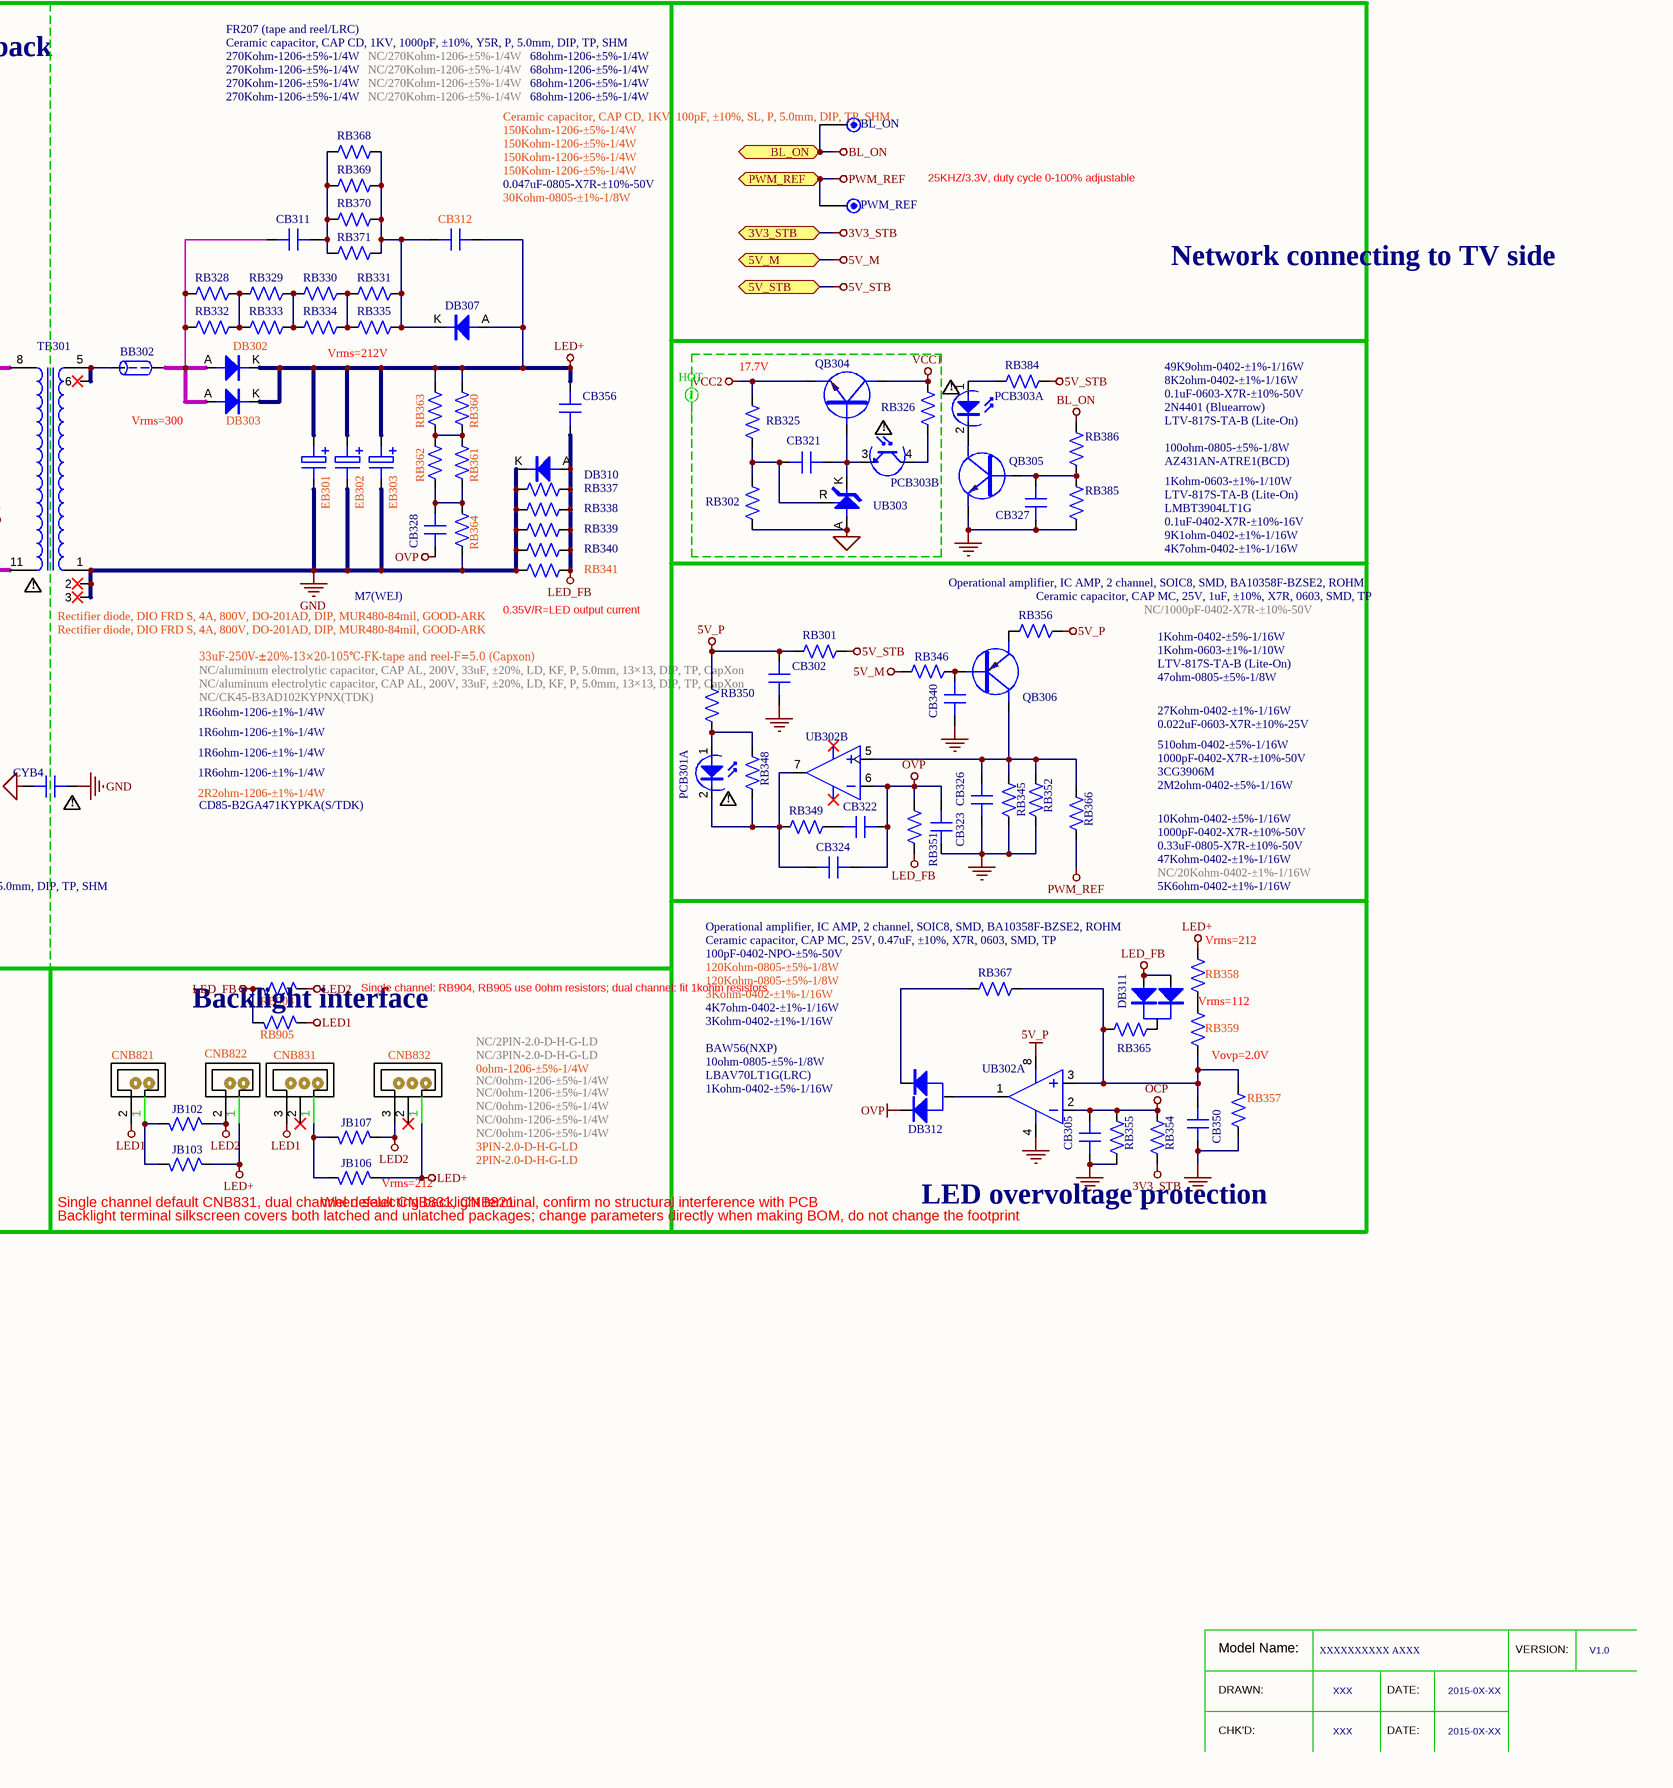
[diagram p0: PCBE84277.SchDoc, bottom right]
# Altium project MISC84277-14.PrjPCB (part 6 of 10)

## Sheet PCBE84277.SchDoc: MISC84277 (continued)

### Library data of the parts
BB101 = φ3.5×6.0×0.65mm-CP(编带/秀益达)-9-DAI: Through-hole ferrite bead
BB201 = Φ3.5×9.0×0.65mm(编带/秀益达)-DLAI: Through-hole ferrite bead
BB301 = φ3.5×6.0×0.65mm-CP(编带/秀益达)-DAI: Through-hole ferrite bead
BB302 = φ3.5×6.0×0.65mm-CP(编带/RY)-DLAI: Through-hole ferrite bead
CB2 CB3 = MPX450K474(散装/日精)-DHMI: CAP(474)
CB101 CB303 CB305 = 100pF-0402-NPO-±5%-50V-D
CB102 CB109 CB206 CB304 CB321 = 0.1uF-0603-X7R-±10%-50V-D: CAP
CB103 CB323 CB324 = 1000pF-0402-X7R-±10%-50V-D
CB110 CB340 = 1000pF-0402-X7R-±10%-50V-D: CAP
CB111 CB112 = 1uF-0805-X7R-±10%-25V-D: CAP
CB113 = 220PF-0805-NPO-±10%-200V-D: CAP
CB114 CB306 = C242G472J20A201(编带/法拉)-DAI: CAP
CB116 CB209 CB316 = 陶瓷电容,CAP CD,1KV,100pF,±10%,SL,P,5.0mm,DIP,TP,SHM-DHAI: CAP
CB118 = 1000pF-0805-NPO-±10%-200V-D: CAP
CB201 = 0.047uF-0603-X7R-±10%-25V-D
CB204 = 陶瓷电容,CAP CD,1KV,4700pF,±20%,Y5U,P,5.0mm,DIP,TP,SHM-DHAI
CB205 = 220pF-0402-NPO-±5%-50V-D
CB211 CB312 = CC45SL3AD470JYPNA(TDK)-DHAI: CAP
CB212 = 0.22uF-0805-X7R-±10%-50V-D
CB221 CB301 = 4700pF-0402-X7R-±10%-50V-D
CB302 = 陶瓷电容,CAP MC,25V,1uF,±10%,X7R,0603,SMD,TP-D: CAP
CB311 = CAP CD,1KV,1000pF,±10%,Y5R,P,5.0mm,DIP,TP,SHM-DHAI: CAP
CB322 = 0.022uF-0603-X7R-±10%-25V-D
CB326 = 0.33uF-0805-X7R-±10%-50V-D: C
CB327 CB951 = 0.1uF-0402-X7R-±10%-16V-D: CAP
CB328 = 0.047uF-0805-X7R-±10%-50V-D
CB350 = 0.47uF-0603-X5R-±10%-16V-D
CB356 = CK45-B3AD102KYPNX(TDK)-DHAI: CAP
CNB1 = 连接插座,connect jack,2Pin,D7.92,L,SNAP,Fool-proofing,nature,L=2.8mm,DIP,AMA-DLMI: AC socket
CNB2 = 2PIN-2.0-D-H-G-B-DHMI: Socket
CNB812 = 2×4PIN-2.0-L-H-F-镀金-LK-DLMI: CN-gold pin
CNB821 CNB822 = 2PIN-2.0-D-H-G-DHMI
CNB831 CNB832 = 3PIN-2.0-D-H-G-DHMI: Socket
CXB1 = X电容,CAP X2,MP,275VAC,0.47uF,±10%,S,15mm-Mini,PC,DIP,BM-DHMI: CAP
CYB1 CYB2 = CD70-B2GA221KYPKA(S/TDK)-DHMI: CAP
CYB3 CYB4 = CD70ZU2GA102MYPKA(S/TDK)-DHMI: CAP
DB1-DB4 = 1N5408G(编带/GOOD-ARK)-DLMI: Diode
DB101 = MBRB10150CT(GOOD-ARK)-D: Diode
DB102 DB204 = LBAV70LT1G(LRC)-D: Diode
DB105 = 1N4007-DO-41-DLAI: Diode
DB106 DB306 DB307 = FR207(编带/LRC)-DLAI: Diode
DB201 = 整流二极管,DIO FRD S,8A,600V,ITO-220AC,DIP,UGF8J C0G,TSC-DHMI: Diode
DB202 DB203 = GS3J-B(GULF)-D: Diode
DB302 DB303 = 整流二极管,DIO FRD S,4A,800V,DO-201AD,DIP,MUR480-84mil,GOOD-ARK-DLMI: Diode
DB310 DB370 DB371 = M7(WEJ)-D: Diode
DB311 DB901 DB951 = LBAV70LT1G(LRC)-D
DB312 = BAW56(NXP)-D
EB101 EB103 = 470uF-25V-±20%-10×12.5-105℃-GF-编带-F=5.0(CapXon)-DHAI: Electrolytic
EB102 = 270uF-16V-±20%-8×11.5-105℃-PS-短脚-F=3.5(Capxon): Solid-state
EB106 = 100uF-35V-±20%-6.3×11-105℃-KF-编带-F=2.5(CapXon)-DHAI: Electrolytic
EB107 = 10uF-50V-±20%-5×11-105℃-GH-编带-F=2.5(CapXon)-DHAI: Electrolytic
EB201 = 100uF-450V-±20%-16×35.5-105℃-KM-折脚(H=8.1mm)(Capxon)-DLMI: Electrolytic
EB301 = 68uF-160V-±20%-12.5×20-105℃-RR-编带-F=5.0(Samxon)-DHMI: Electrolytic
EB302 EB303 = 铝电解电容,CAP AL,200V,33uF,±20%,LD,KF,P,5.0mm,13×13,DIP,TP,CapXon-DHAI: Electrolytic
EVA1-EVA7 = 7×7×3mm-C-4305防火泡棉-黑色-DLMI: EVA
FB1 = 2010T3.15A250VA1(编带/华德)-DHAI: FUSE
GD1-GD4 = 7.00×8.54mm-尼龙-白色-DHMI
GL1-GL4 = SLD-8854W-白胶: White glue
HSB2 = 40×25×5.0-黑色-带引脚(厚=1.5mm)-FR-DLMI: Heatsink
HSB3 = 50×25×5.0-黑色-带引脚(厚=1.5mm)-FR-DLMI: Heatsink
HSB6 = 17.5×14.5×0.5-本色-Cu-MRD-D: Heatsink
JB102 JB103 JB106 JB107 RB904 RB905 = 0ohm-1206-±5%-1/4W-D: RES
LB1 = SYDR1212-L003-EDL-DHMI: I-shaped inductor
LB202 = SYEQ2612-L250uA-SQ-DLMI: PFC inductor
LCB1 = SYT10-L002-SQ-DHMI: Common mode
LCB2 = SYT14-L003-JM-DLMI: Common mode
MB1 MB2 = PM3.0×8.0×5.5mm-银色-双垫片-DHMI: SCREW
ML1 = MALAY
MOVB1 = TVR10561KSC3AGGW(短脚/为勤)-DHMI: Varistor
NTCB2 = SCK102R55AMBY502(短脚/为勤)-DHMI: Thermistor
PCB101 = LTV-817S-TA-B(光宝)-DMI: Optocoupler
PCB301 PCB303 = LTV-817S-TA-B(光宝)-D: Optocoupler
QB101 = 场效应管,NMOS,5A,700V,0.9ohm@ID=2.5A@VGS=10V,TO-252,MMD70R900PRH,MAGNACHIP-D: N Channel Single MOSFET
QB102 QB302 QB306 = 3CG3906M-D: Transistor
QB201 = TK15A50D(东芝)-DLMI: MOS
QB201和散热片之间 QB301和散热片之间 = 0.05g-导热硅脂: Thermal grease
QB301 = MDF7N65BTH(Magnachip)-DLMI: MOS
QB304 = 2N4401(蓝箭)-DAI
QB305 QB951 = LMBT3904LT1G-D-NPN: Q-NPN-#-#-#
QB911 QB921 QB931 QB941 = 2SD1857L-Q-T9N-B(UTC)-DAI: Transistor
RB1-RB4 = 1M2ohm-1206-±5%-1/4W-D: RES
RB101 RB102 = 330Kohm-1206-±5%-1/4W-D: RES
RB103 = 10Kohm-0402-±1%-1/16W-D
RB104 RB226 RB366 = 47Kohm-0402-±1%-1/16W-D
RB105 RB107 RB215 RB305 RB307 RB346 = 510ohm-0402-±5%-1/16W-D
RB106 RB365 = 68ohm-0805-±5%-1/8W-D
RB108 RB213 RB308 = 20ohm-0805-±5%-1/8W-D: RES
RB109 RB214 RB225 RB309 = 10Kohm-0402-±5%-1/16W-D: RES
RB110 RB114-RB118 RB210 RB314 RB315 RB911-RB913 RB921-RB923 RB931-RB933 RB941-RB943 = 10ohm-1206-±5%-1/4W-D: RES
RB123 RB124 = 47ohm-1206-±5%-1/4W-D: RES
RB131 = 2Kohm-0603-±5%-1/10W-D
RB132 RB133 = 3Kohm-0402-±5%-1/16W-D: RES
RB134 = 4K7ohm-0402-±1%-1/16W-D: RES
RB135 = 18Kohm-0402-±1%-1/16W-D: RES
RB141 RB142 = 2Mohm-1206-±5%-1/4W-D: RES
RB143 = 0ohm-0402-±5%-1/16W-D
RB144-RB147 RB317-RB324 = 100Kohm-1206-±5%-1/4W-D: RES
RB148 RB310 = MOF-0R27ohm-±5%-2WS(编带/Futaba)-DLAI: RES
RB201-RB204 = 1Mohm-1206-±1%-1/4W-D: RES
RB205 = 560kohm-0402-±1%-1/16W-D
RB206 RB349 = 27Kohm-0402-±1%-1/16W-D: RES
RB209 = 39Kohm-0805-±1%-1/8W-D: RES
RB212 RB301 RB306 = 47ohm-0805-±5%-1/8W-D: RES
RB217 = MOF-0R1ohm-±5%-2WS(编带/Futaba)-DLAI: RES
RB218 = 1R6ohm-1206-±1%-1/4W-D: RES
RB219 RB220 = 100ohm-1206-±5%-1/4W-D: RES
RB221 = 1Kohm-0402-±5%-1/16W-D
RB223 RB224 RB391 RB392 = 22ohm-1206-±5%-1/4W-D
RB227 = 0ohm-0402-±5%-1/16W-D: RES
RB302 = 8K2ohm-0402-±1%-1/16W-D
RB303 RB351 = 10Kohm-0402-±5%-1/16W-D
RB304 = 47Kohm-0402-±5%-1/16W-D
RB325 = 49K9ohm-0402-±1%-1/16W-D
RB326 = 1Kohm-0805-±5%-1/8W-D: R
RB328-RB332 RB334 RB335 = 270Kohm-1206-±5%-1/4W-D
RB333 = 200Kohm-1206-±5%-1/4W-D: RES
RB337 RB339 RB340 = 4R7ohm-1206-±1%-1/4W-D: RES
RB338 = 8R2ohm-1206-±5%-1/4W-D: RES
RB341 = 2R2ohm-1206-±1%-1/4W-D: RES
RB345 = 5K6ohm-0402-±1%-1/16W-D: RES
RB347 = MOF-300Kohm-±5%-2WS(编带/Futaba)-DLAI: RES
RB348 RB367 = 1Kohm-0402-±5%-1/16W-D: RES
RB350 RB384 = 1Kohm-0603-±1%-1/10W-D
RB352 = 20Kohm-0402-±1%-1/16W-D: RES
RB354 = 2Kohm-0402-±1%-1/16W-D: RES
RB355 = 3K9ohm-0402-±1%-1/16W-D
RB356 = 2M2ohm-0402-±5%-1/16W-D
RB357 = 3Kohm-0402-±1%-1/16W-D
RB358 RB359 = 150Kohm-0805-±1%-1/8W-D: RES
RB360-RB363 = 150Kohm-1206-±5%-1/4W-D: RES
RB364 = 30Kohm-0805-±1%-1/8W-D
RB368-RB371 = 68ohm-1206-±5%-1/4W-D: RES
RB385 = 4K7ohm-0402-±1%-1/16W-D
RB386 = 9K1ohm-0402-±1%-1/16W-D
RB901-RB903 = 470ohm-1206-±5%-1/4W-D: RES
RB951 = 2Kohm-0402-±1%-1/16W-D
RB952 = 20Kohm-1206-±5%-1/4W-D
TB101 = SYEQ2612-T012A-YX-DLMI: Transformer
TB301 = SYEFD30-T009-XX-DLMI: Transformer
TP-TDT = TEST
UB101 UB301 = LD5530 RGL(通嘉)-D: IC
UB102 UB303 = AZ431AN-ATRE1(BCD)-D: SMD 431
UB201 = PWM控制器,IC PWM Controller,300KHz,SOP-8,SMD,FAN7930CMX_G,Fairchild-D: IC
UB302 = 运算放大器,IC AMP,2 channel,SOIC8,SMD,BA10358F-BZSE2,ROHM-D: Operational Amplifier
ZDB101 = BZX84C24(蓝箭)-D: Diode